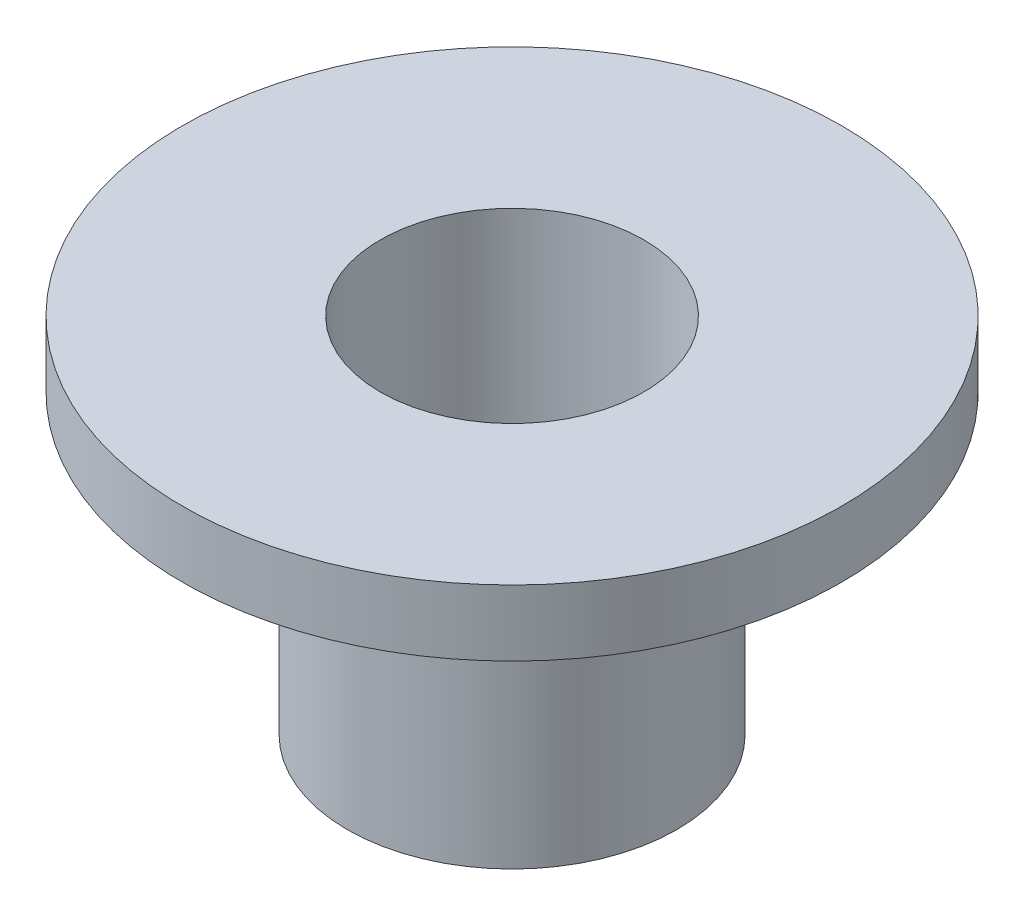
SolidWorks part; units mm, degrees
ref_plane "Front Plane" through (0, 0, 0) normal (0, 0, 1) x (1, 0, 0)
ref_plane "Top Plane" through (0, 0, 0) normal (0, 1, 0) x (1, 0, 0)
ref_plane "Right Plane" through (0, 0, 0) normal (1, 0, 0) x (0, 0, -1)
sketch "Sketch1" plane through (0, 0, 0) normal (0, 0, 1) x (1, 0, 0)
  line L0 (0, 0) -> (0, 9) construction
  line L1 (2, 5.5) -> (5, 5.5)
  line L2 (5, 5.5) -> (5, 4.5)
  line L3 (5, 4.5) -> (2.5, 4.5)
  line L4 (2.5, 4.5) -> (2.5, 0)
  line L5 (2.5, 0) -> (2, 0)
  line L6 (2, 5.5) -> (2, 0)
  dimension "D1" = 2
  dimension "D2" = 2.5
  dimension "D3" = 4.5
  dimension "D4" = 1
  dimension "D5" = 5
revolve "Revolve1" add sketch "Sketch1" angle 360 about L0
